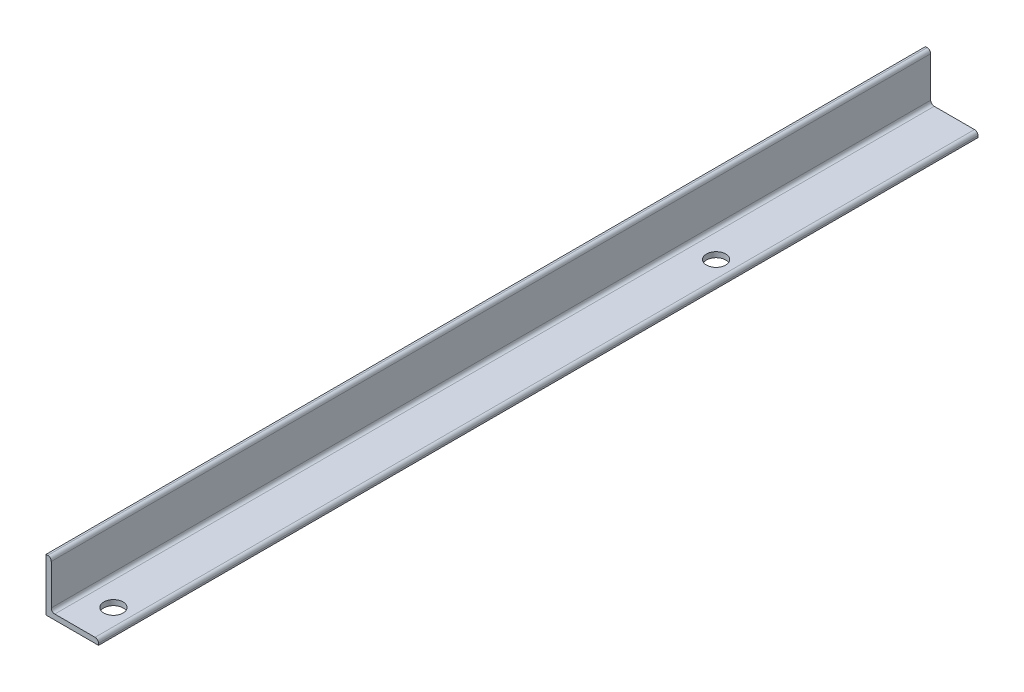
SolidWorks part; units mm, degrees
material "Plain Carbon Steel"
ref_plane "Front Plane" through (0, 0, 0) normal (0, 0, 1) x (1, 0, 0)
ref_plane "Top Plane" through (0, 0, 0) normal (0, 1, 0) x (1, 0, 0)
ref_plane "Right Plane" through (0, 0, 0) normal (1, 0, 0) x (0, 0, -1)
sketch "Sketch1" plane through (0, 0, 0) normal (0, 0, 1) x (1, 0, 0)
  line L0 (0, 0) -> (30, 0)
  line L1 (0, 0) -> (0, 30)
  line L2 (5, 3) -> (28, 3)
  line L3 (3, 5) -> (3, 28)
  line L4 (0, 30) -> (1, 30)
  line L5 (30, 1) -> (30, 0)
  line L6 (3, 3) -> (3, 30) construction
  line L7 (3, 3) -> (30, 3) construction
  arc A0 (1, 30) -> (3, 28) centre (1, 28) cw
  arc A1 (5, 3) -> (3, 5) centre (5, 5) cw
  arc A2 (30, 1) -> (28, 3) centre (28, 1) ccw
  dimension "D3" = 2
  dimension "D1" = 30
  dimension "D2" = 3
extrude "Boss-Extrude1" add sketch "Sketch1" along normal blind 502
sketch "Sketch2" plane through (0, 0, 0) normal (0, -1, 0) x (1, 0, 0)
  line L0 (0, 502) -> (30, 502) construction
  line L1 (0, 502) -> (0, 0) construction
  circle A0 centre (18.5, 482) radius 5.5
  dimension "D3" = 11
  dimension "D1" = 20
  dimension "D2" = 18.5
extrude "Cut-Extrude1" cut sketch "Sketch2" against normal blind 3
pattern_linear "LPattern1" count 2 spacing 344 along (0, 0, -1) of "Cut-Extrude1"
